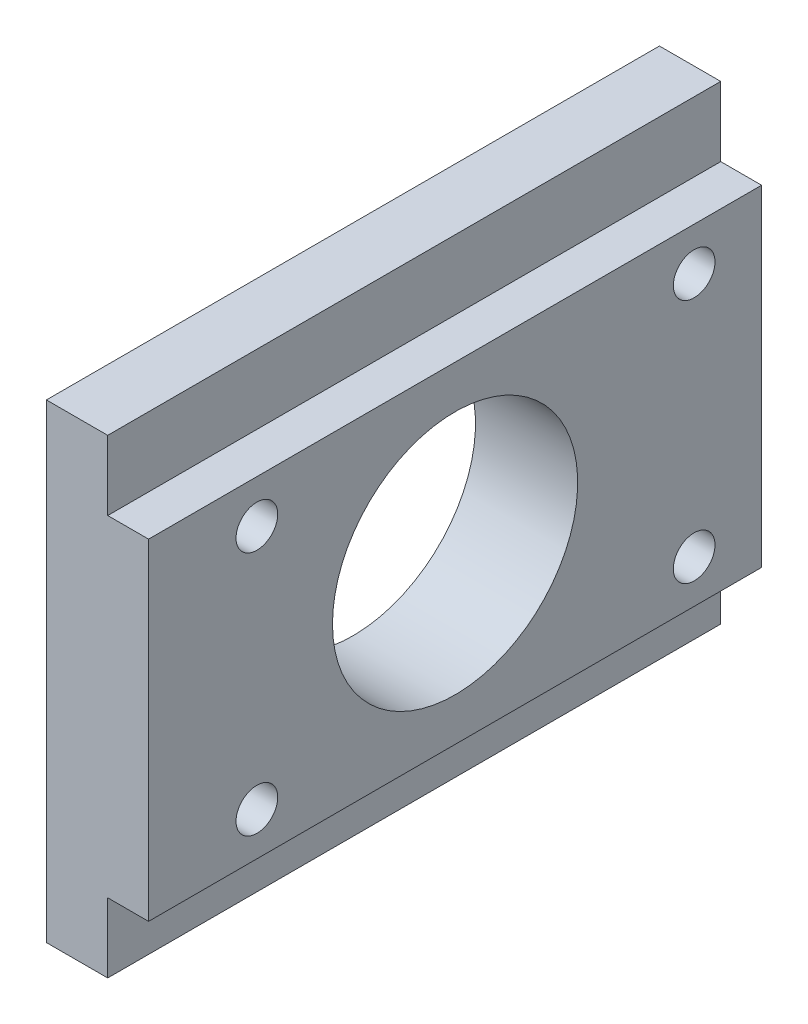
SolidWorks part; units mm, degrees
ref_plane "前视基准面" through (0, 0, 0) normal (0, 0, 1) x (1, 0, 0)
ref_plane "上视基准面" through (0, 0, 0) normal (0, 1, 0) x (1, 0, 0)
ref_plane "右视基准面" through (0, 0, 0) normal (1, 0, 0) x (0, 0, -1)
other "Configuration Table"
sketch "草图1" plane through (0, 0, 0) normal (0, 0, 1) x (1, 0, 0)
  line L0 (0, 0) -> (56.2791, 0) construction
  line L1 (0, 57.5) -> (0, -57.5)
  line L2 (0, -57.5) -> (15, -57.5)
  line L3 (15, -57.5) -> (15, -40.5)
  line L4 (15, -40.5) -> (25, -40.5)
  line L5 (25, -40.5) -> (25, 40.5)
  line L6 (15, 40.5) -> (25, 40.5)
  line L7 (15, 57.5) -> (15, 40.5)
  line L8 (0, 57.5) -> (15, 57.5)
  point P9 (25, 0)
  dimension "D1" = 57.5
  dimension "D2" = 25
  dimension "D3" = 15
  dimension "D4" = 17
extrude "凸台-拉伸1" add sketch "草图1" along normal mid plane 150
sketch "草图2" plane through (0, 0, 0) normal (-1, 0, 0) x (0, 0, 1)
  circle A0 centre (0, 0) radius 30
  dimension "D1" = 60
extrude "切除-拉伸1" cut sketch "草图2" against normal blind 210
sketch "草图5" plane through (0, 0, 0) normal (-1, 0, 0) x (0, 0, 1)
  line L0 (-58.5, 30) -> (48.5, 30) construction
  line L1 (-58.5, 30) -> (-58.5, -30) construction
  point P0 (-58.5, 30)
  point P10 (48.5, 30)
  point P11 (48.5, -30)
  point P12 (-58.5, -30)
  dimension "D1" = 30
  dimension "D2" = 58.5
  dimension "D5" = 107
  dimension "D6" = 60
  dimension "D3" = 2
  dimension "D4" = 2
hole_wizard "M12 螺纹孔1" positions "草图5" profile "草图4" tap size "M12" standard "GB" end condition up to next
sketch "草图4" plane through (0, 30, -58.5) normal (0, 1, 0) x (0, 0, 1)
  line L0 (0, 0) -> (0, 25)
  line L1 (0, 25) -> (5.1, 25)
  line L2 (5.1, 25) -> (5.1, 0)
  line L5 (5.1, 0) -> (0, 0)
  line L11 (0, -6.35) -> (0, 107.95) construction
  dimension "通孔螺纹孔钻头直径" = 10.2
  dimension "通孔螺纹孔钻头深度" = 25
cosmetic thread "孔螺纹线1" parameters "D2"=12
cosmetic thread "孔螺纹线2" parameters "D2"=12
cosmetic thread "孔螺纹线3" parameters "D2"=12
cosmetic thread "孔螺纹线4" parameters "D2"=12
